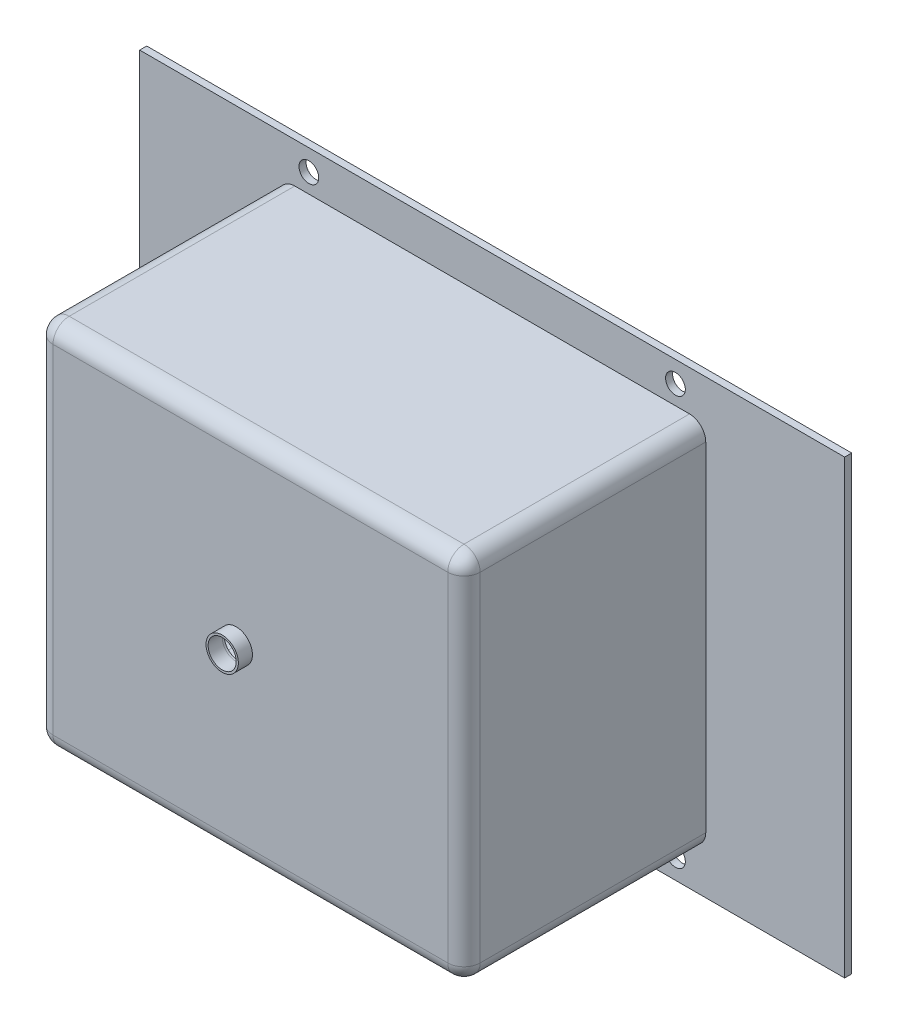
from build123d import *

# Parameters (mm, degrees)
SKETCH1_W           = 500
SKETCH1_H           = 320
SKETCH1_W_2         = 300
SKETCH1_H_2         = 260
BOSS_EXTRUDE1_DEPTH = 5
SKETCH2_W           = 303
SKETCH2_H           = 263
SKETCH2_W_2         = 300
SKETCH2_H_2         = 260
BOSS_EXTRUDE2_DEPTH = 170
SKETCH3_W           = 303
SKETCH3_H           = 263
SKETCH3_R           = 10
BOSS_EXTRUDE3_DEPTH = 1.5
FILLET2_R           = 10
FILLET3_R           = 11.5
SKETCH4_R           = 11.467682252
SKETCH4_R_2         = 9.967682252
BOSS_EXTRUDE4_DEPTH = 10
SKETCH5_R           = 7
CUT_EXTRUDE1_DEPTH  = 529.093031577
SKETCH6_R           = 10.66612067
BOSS_EXTRUDE5_DEPTH = 2


with BuildPart() as part:
    # Sketch1 → Boss-Extrude1 (new body)
    with BuildSketch(Plane.XY):
        with Locations((150, 130)):
            Rectangle(SKETCH1_W, SKETCH1_H)
        with Locations((150, 130)):
            Rectangle(SKETCH1_W_2, SKETCH1_H_2, mode=Mode.SUBTRACT)
    extrude(amount=BOSS_EXTRUDE1_DEPTH)

    # Sketch2 → Boss-Extrude2 (add)
    with BuildSketch(Plane.XY.offset(5)):
        with Locations((150, 130)):
            Rectangle(SKETCH2_W, SKETCH2_H)
        with Locations((150, 130)):
            Rectangle(SKETCH2_W_2, SKETCH2_H_2, mode=Mode.SUBTRACT)
    extrude(amount=BOSS_EXTRUDE2_DEPTH)

    # Sketch3 → Boss-Extrude3 (add)
    with BuildSketch(Plane.XY.offset(175)):
        with Locations((150, 130)):
            Rectangle(SKETCH3_W, SKETCH3_H)
        with Locations((140, 130)):
            Circle(SKETCH3_R, mode=Mode.SUBTRACT)
    extrude(amount=BOSS_EXTRUDE3_DEPTH)

    # Fillet2
    fillet2_edges = [part.edges().sort_by_distance(p)[0] for p in [
        (0, 260, 87.5),
        (0, 0, 87.5),
        (300, 0, 87.5),
        (300, 260, 87.5),
        (0, 130, 175),
        (150, 0, 175),
        (300, 130, 175),
        (150, 260, 175),
    ]]
    fillet(fillet2_edges, radius=FILLET2_R)

    # Fillet3
    fillet3_edges = [part.edges().sort_by_distance(p)[0] for p in [
        (-1.5, 261.5, 90.75),
        (-1.5, -1.5, 90.75),
        (301.5, -1.5, 90.75),
        (301.5, 261.5, 90.75),
        (301.5, 130, 176.5),
        (150, 261.5, 176.5),
        (-1.5, 130, 176.5),
        (150, -1.5, 176.5),
    ]]
    fillet(fillet3_edges, radius=FILLET3_R)

    # Sketch4 → Boss-Extrude4 (add)
    with BuildSketch(Plane.XY.offset(176.5)):
        with Locations(Location((140, 130, 0), (0, 0, 180))):
            Circle(SKETCH4_R)
        with Locations((140, 130)):
            Circle(SKETCH4_R_2, mode=Mode.SUBTRACT)
    extrude(amount=BOSS_EXTRUDE4_DEPTH)

    # Sketch5 → Cut-Extrude1 (cut, through all)
    with BuildSketch(Plane(origin=(0, 0, 0), x_dir=(-1, 0, 0), z_dir=(0, 0, -1))):
        with Locations((-20, -15)):
            Circle(SKETCH5_R)
        with Locations((-280, -15)):
            Circle(SKETCH5_R)
        with Locations((-20, 275)):
            Circle(SKETCH5_R)
        with Locations((-280, 275)):
            Circle(SKETCH5_R)
    extrude(amount=-CUT_EXTRUDE1_DEPTH, mode=Mode.SUBTRACT)

    # Sketch6 → Boss-Extrude5 (add)
    with BuildSketch(Plane(origin=(0, 0, 0), x_dir=(-1, 0, 0), z_dir=(0, 0, -1))):
        with Locations(Location((56.636018442, 245.08861857, 0), (0, 0, 180))):
            Circle(SKETCH6_R)
        with Locations(Location((56.636018442, 210.08861857, 0), (0, 0, 180))):
            Circle(SKETCH6_R)
        with Locations(Location((56.636018442, 175.08861857, 0), (0, 0, 180))):
            Circle(SKETCH6_R)
    extrude(amount=BOSS_EXTRUDE5_DEPTH)


solid = part.part
